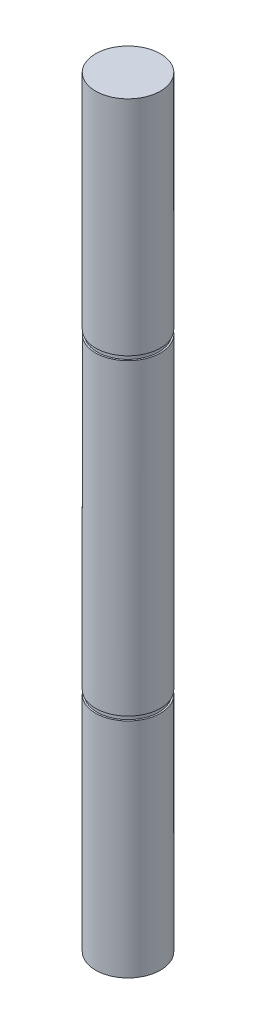
SolidWorks part; units mm, degrees
ref_plane "前视基准面" through (0, 0, 0) normal (0, 0, 1) x (1, 0, 0)
ref_plane "上视基准面" through (0, 0, 0) normal (0, 1, 0) x (1, 0, 0)
ref_plane "右视基准面" through (0, 0, 0) normal (1, 0, 0) x (0, 0, -1)
sketch "草图1" plane through (0, 0, 0) normal (0, 1, 0) x (1, 0, 0)
  circle A0 centre (0, 0) radius 10
  dimension "D1" = 20
extrude "凸台-拉伸1" add sketch "草图1" along normal blind 235
ref_plane "基准面1" through (0, 0, -10) normal (0, 0, -1) x (-1, 0, 0)
ref_plane "基准面3" through (0, 70, 0) normal (0, -1, 0) x (-1, 0, 0)
sketch "草图7" plane through (0, 70, 0) normal (0, -1, 0) x (-1, 0, 0)
  circle A0 centre (0, 0) radius 10 construction
  circle A1 centre (0, 0) radius 10
  circle A2 centre (0, 0) radius 9.5
  dimension "D1" = 19
extrude "切除-拉伸3" cut sketch "草图7" along normal blind 1.3
ref_plane "基准面4" through (0, 165, 0) normal (0, 1, 0) x (1, 0, 0)
sketch "草图8" plane through (0, 165, 0) normal (0, 1, 0) x (1, 0, 0)
  circle A0 centre (0, 0) radius 10 construction
  circle A1 centre (0, 0) radius 10
  circle A2 centre (0, 0) radius 9.5
  dimension "D1" = 19
extrude "切除-拉伸4" cut sketch "草图8" along normal blind 1.3
chamfer "倒角1" [suppressed] distance 0.5 angle 45
ref_plane "基准面2" through (0, 65, 0) normal (0, -1, 0) x (-1, 0, 0)
sketch "MyToolsJD" plane through (0, 0, 0) normal (0, -1, 0) x (-1, 0, 0)
  line L0 (0, 0) -> (10, 0) construction
  line L1 (0, 0) -> (0, 10) construction
  circle A0 centre (0, 0) radius 10 construction
  circle A1 centre (0, 0) radius 10 construction
  dimension "D1" = 90
ref_plane "基准面11" through (0, 0, -10) normal (0, 0, -1) x (-1, 0, 0)
sketch "MyToolsZJC" plane through (0, 0, -10) normal (0, 0, -1) x (0, 1, 0)
  line L0 (115.5, 0) -> (119.5, 0) construction
  line L1 (115.5, 3) -> (119.5, 3)
  line L2 (115.5, -3) -> (119.5, -3)
  line L3 (0, 0) -> (115.5, 0) construction
  line L5 (117.5, 10) -> (117.5, -35.6075) construction
  line L6 (165, 10) -> (70, 10) construction
  arc A0 (115.5, 3) -> (115.5, -3) centre (115.5, 0) ccw
  arc A1 (119.5, -3) -> (119.5, 3) centre (119.5, 0) ccw
  point P2 (117.5, 0)
  point P13 (122.5, 0)
  point P14 (112.5, 0)
  dimension "D3" = 10
  dimension "D1" = 6
extrude "ZJCQC" cut sketch "MyToolsZJC" against normal blind 3.5
